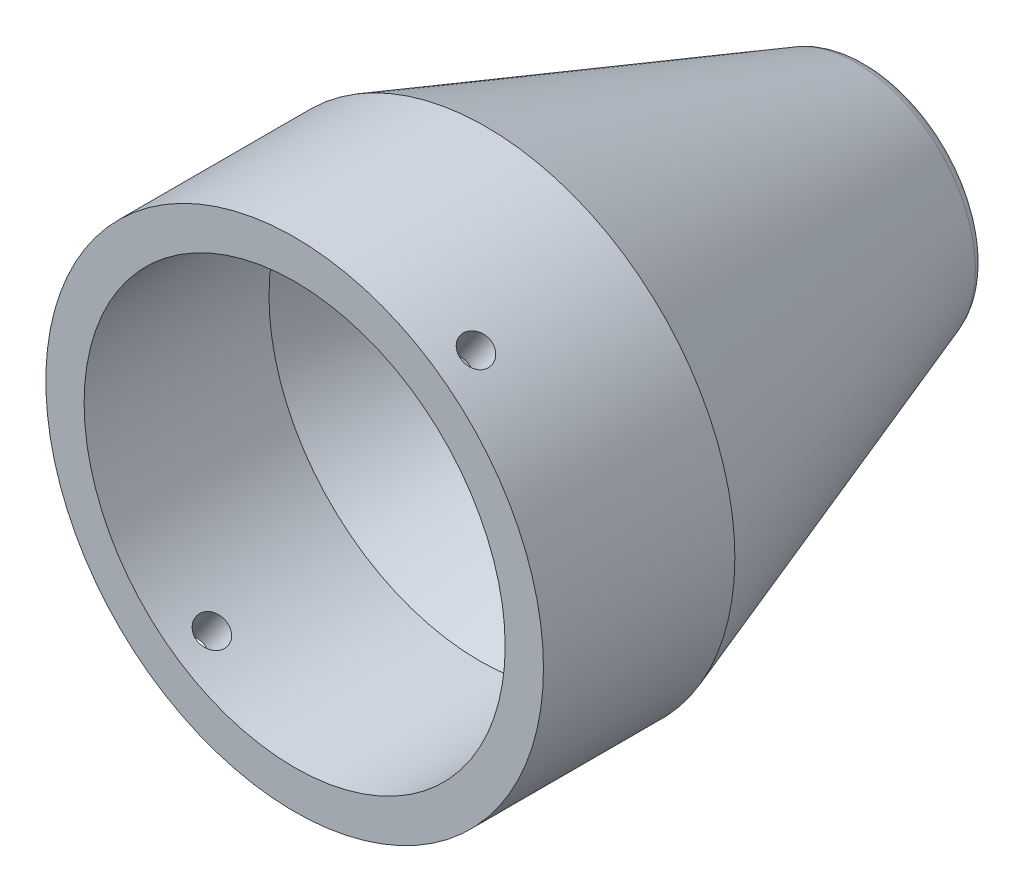
from build123d import *

# Parameters (mm, degrees)
M100_CLEARANCE_HOLE1_D       = 110
M100_CLEARANCE_HOLE1_DEPTH   = 48.300542714
M100_CLEARANCE_HOLE1_TIP     = 157.142859071
F_8_0_8_DIAMETER_HOLE1_D     = 8
F_8_0_8_DIAMETER_HOLE1_DEPTH = 140.145647392
FILLET1_R                    = 5


with BuildPart() as part:
    # Sketch1 → Revolve1 (revolve)
    with BuildSketch(Plane(origin=(0, 234.743963655, 0), x_dir=(1, 0, 0), z_dir=(0, 1, 0))):
        Polygon((551.230642584, 1664.998443067), (521.230642584, 1664.998443067), (521.230642584, 1514.998443067), (586.230642584, 1514.998443067), (586.230642584, 1564.998443067), align=None)
    revolve(axis=Axis((521.230642584, 234.743963655, -1664.998443067), (0, 0, 1)))

    # M100 clearance hole1
    with Locations(Plane.XY.offset(-1514.998443067)):
        with Locations((521.230642584, 234.743963655)):
            Hole(M100_CLEARANCE_HOLE1_D / 2, depth=M100_CLEARANCE_HOLE1_DEPTH)
            with Locations((0, 0, -(M100_CLEARANCE_HOLE1_DEPTH + M100_CLEARANCE_HOLE1_TIP / 2))):  # 38.580092° drill point
                Cone(0, M100_CLEARANCE_HOLE1_D / 2, M100_CLEARANCE_HOLE1_TIP, mode=Mode.SUBTRACT)

    # Ø8.0 (8) diameter hole1
    with Locations(Plane(origin=(558.630703666, 287.906313406, -1524.998443067), x_dir=(0.817882303865, -0.575385555106, 0), z_dir=(0.575385555106, 0.817882303865, 0))):
        with Locations((0, 0)):
            Hole(F_8_0_8_DIAMETER_HOLE1_D / 2, depth=F_8_0_8_DIAMETER_HOLE1_DEPTH)

    # Fillet1
    fillet1_edges = [part.edges().sort_by_distance(p)[0] for p in [
        (491.230642584, 234.743963655, -1664.998443067),
    ]]
    fillet(fillet1_edges, radius=FILLET1_R)


solid = part.part
